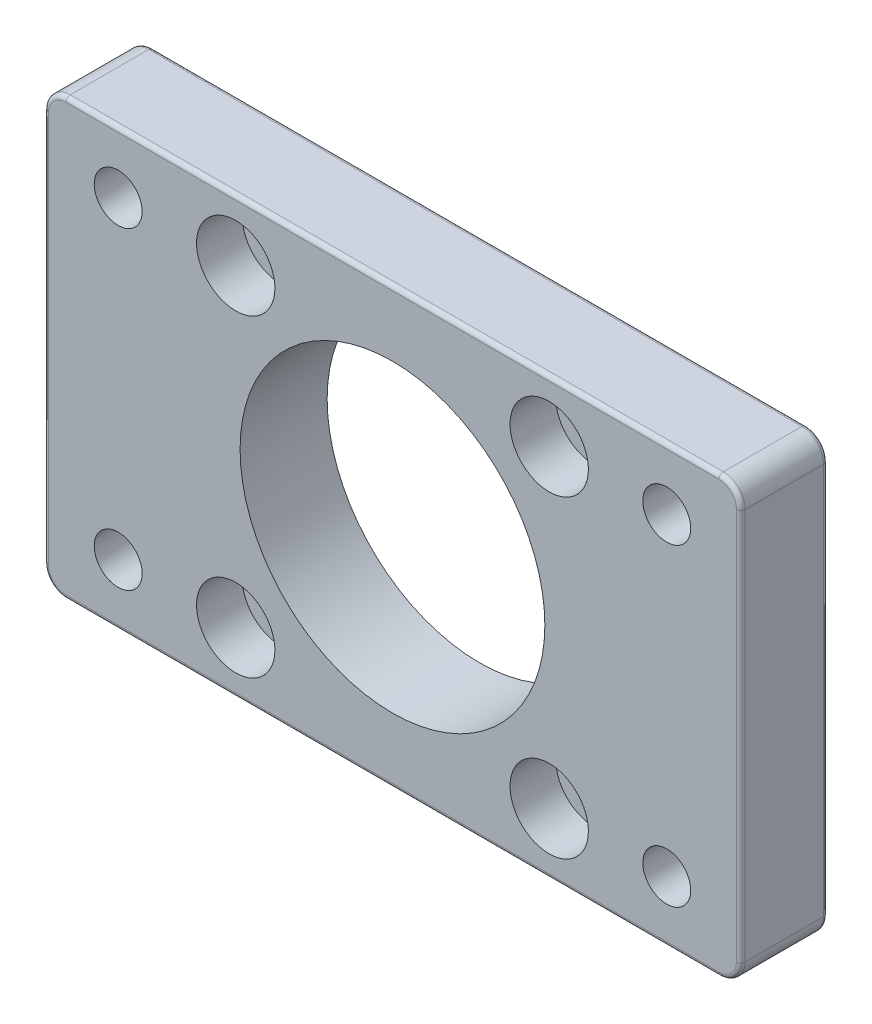
from build123d import *

# Parameters (mm, degrees)
SKETCH1_W                                           = 160
SKETCH1_H                                           = 100
SKETCH1_R                                           = 35
BOSS_EXTRUDE1_DEPTH                                 = 20
FILLET1_R                                           = 5
HOLE_SPEC_PER_SOCKET_HEAD_CAP_SCREW_TYP_D           = 11
HOLE_SPEC_PER_SOCKET_HEAD_CAP_SCREW_TYP_CBORE_D     = 18
HOLE_SPEC_PER_SOCKET_HEAD_CAP_SCREW_TYP_CBORE_DEPTH = 10.5
HOLE_SPEC_PER_SOCKET_HEAD_CAP_SCREW_2_D             = 11
HOLE_SPEC_PER_SOCKET_HEAD_CAP_SCREW_2_CBORE_D       = 18
HOLE_SPEC_PER_SOCKET_HEAD_CAP_SCREW_2_CBORE_DEPTH   = 11
FILLET2_R                                           = 1


with BuildPart() as part:
    # Sketch1 → Boss-Extrude1 (new body)
    with BuildSketch(Plane.XY):
        Rectangle(SKETCH1_W, SKETCH1_H)
        Circle(SKETCH1_R, mode=Mode.SUBTRACT)
    extrude(amount=BOSS_EXTRUDE1_DEPTH)

    # Fillet1
    fillet1_edges = [part.edges().sort_by_distance(p)[0] for p in [
        (-80, 50, 10),
        (80, 50, 10),
        (80, -50, 10),
        (-80, -50, 10),
    ]]
    fillet(fillet1_edges, radius=FILLET1_R)

    # Hole Spec _per socket head cap screw typ (through all)
    with Locations(Plane.XY.offset(20)):
        with Locations((-36, 36), (36, 36), (-36, -36), (36, -36)):
            CounterBoreHole(HOLE_SPEC_PER_SOCKET_HEAD_CAP_SCREW_TYP_D / 2, HOLE_SPEC_PER_SOCKET_HEAD_CAP_SCREW_TYP_CBORE_D / 2, HOLE_SPEC_PER_SOCKET_HEAD_CAP_SCREW_TYP_CBORE_DEPTH)

    # Hole Spec _per socket head cap screw 2 (through all)
    with Locations(Plane(origin=(0, 0, 0), x_dir=(-1, 0, 0), z_dir=(0, 0, -1))):
        with Locations((-63, 36), (63, 36), (-63, -36), (63, -36)):
            CounterBoreHole(HOLE_SPEC_PER_SOCKET_HEAD_CAP_SCREW_2_D / 2, HOLE_SPEC_PER_SOCKET_HEAD_CAP_SCREW_2_CBORE_D / 2, HOLE_SPEC_PER_SOCKET_HEAD_CAP_SCREW_2_CBORE_DEPTH)

    # Fillet2
    fillet2_edges = [part.edges().sort_by_distance(p)[0] for p in [
        (80, 0, 0),
        (80, 0, 20),
        (-80, 0, 0),
        (0, 50, 0),
        (0, -50, 0),
        (78.535533906, 48.535533906, 0),
        (-78.535533906, 48.535533906, 0),
        (-78.535533906, -48.535533906, 0),
        (78.535533906, -48.535533906, 0),
        (0, -50, 20),
        (-80, 0, 20),
        (0, 50, 20),
        (78.535533906, 48.535533906, 20),
        (-78.535533906, 48.535533906, 20),
        (-78.535533906, -48.535533906, 20),
        (78.535533906, -48.535533906, 20),
    ]]
    fillet(fillet2_edges, radius=FILLET2_R)


solid = part.part
